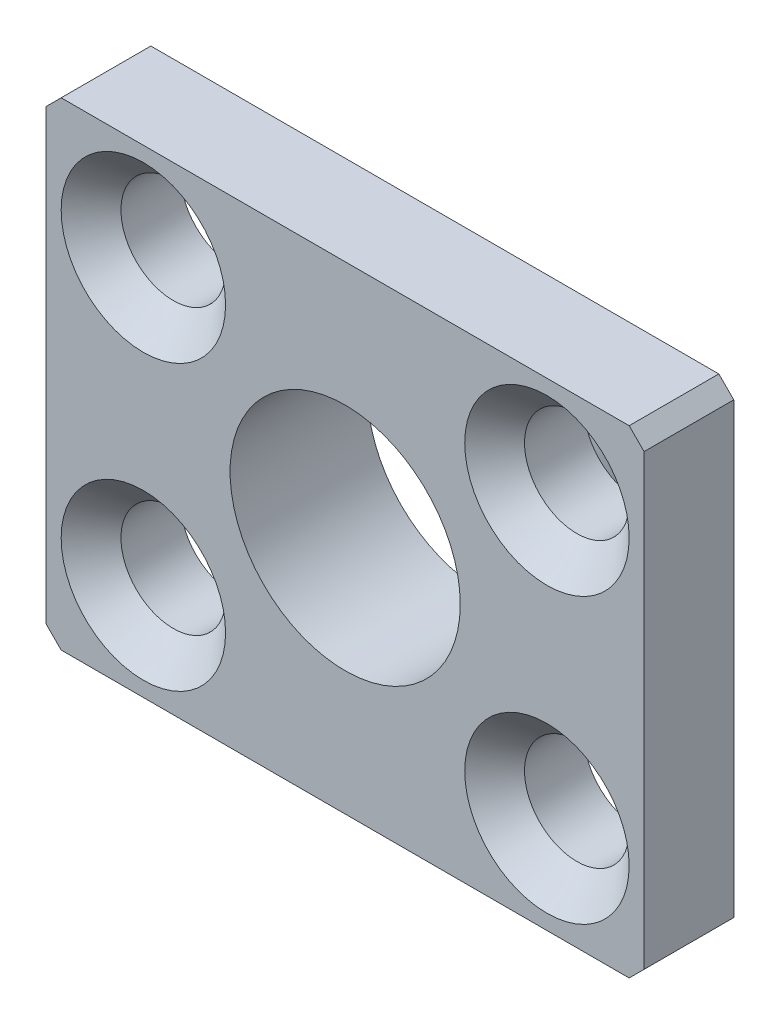
SolidWorks part; units mm, degrees
ref_plane "Front Plane" through (0, 0, 0) normal (0, 0, 1) x (1, 0, 0)
ref_plane "Top Plane" through (0, 0, 0) normal (0, 1, 0) x (1, 0, 0)
ref_plane "Right Plane" through (0, 0, 0) normal (1, 0, 0) x (0, 0, -1)
sketch "Sketch1" plane through (0, 0, 0) normal (0, 0, 1) x (1, 0, 0)
  circle A0 centre (0, 0) radius 3.85
  circle A1 centre (0, 0) radius 5.45
  dimension "D1" = 7.7
  dimension "D2" = 10.9
extrude "Boss-Extrude1" add sketch "Sketch1" along normal blind 1.6
sketch "Sketch2" plane through (0, 0, 1.6) normal (0, 0, 1) x (1, 0, 0)
  line L1 (-10, 8) -> (10, 8)
  line L2 (-10, 8) -> (-10, -8)
  line L3 (-10, -8) -> (10, -8)
  line L4 (10, 8) -> (10, -8)
  line L5 (-10, 8) -> (10, -8) construction
  line L6 (-10, -8) -> (10, 8) construction
  line L11 (-6.055, 4.2609) -> (6.75, -4.75) construction
  line L12 (-6.75, 4.75) -> (6.75, 4.75) construction
  line L13 (-6.75, 4.75) -> (-6.75, -4.75) construction
  line L14 (-6.75, -4.75) -> (6.75, -4.75) construction
  line L15 (6.75, 4.75) -> (6.75, -4.75) construction
  line L16 (-6.75, 4.75) -> (6.75, -4.75) construction
  line L17 (-6.75, -4.75) -> (6.75, 4.75) construction
  circle A0 centre (0, 0) radius 3.85 construction
  circle A1 centre (0, 0) radius 3.85
  circle A2 centre (-6.75, 4.75) radius 1.75
  circle A3 centre (-6.75, -4.75) radius 1.75
  circle A4 centre (6.75, -4.75) radius 1.75
  circle A5 centre (6.75, 4.75) radius 1.75
  point P0 (0, 0)
  point P5 (0, 0)
  dimension "D3" = 3.5
  dimension "D1" = 20
  dimension "D2" = 16
  dimension "D4" = 13.5
  dimension "D5" = 9.5
extrude "Boss-Extrude2" add sketch "Sketch2" along normal blind 3
chamfer "Chamfer1" distance 0.3 angle 45 1 edges at (5.45, 0, 0)
chamfer "Chamfer2" distance 1 angle 45 4 edges at (8.5, -4.75, 4.6) (-5, -4.75, 4.6) (8.5, 4.75, 4.6) (-5, 4.75, 4.6)
chamfer "Chamfer3" distance 0.5 angle 45 4 edges at (-10, -8, 3.1) (10, -8, 3.1) (10, 8, 3.1) (-10, 8, 3.1)
